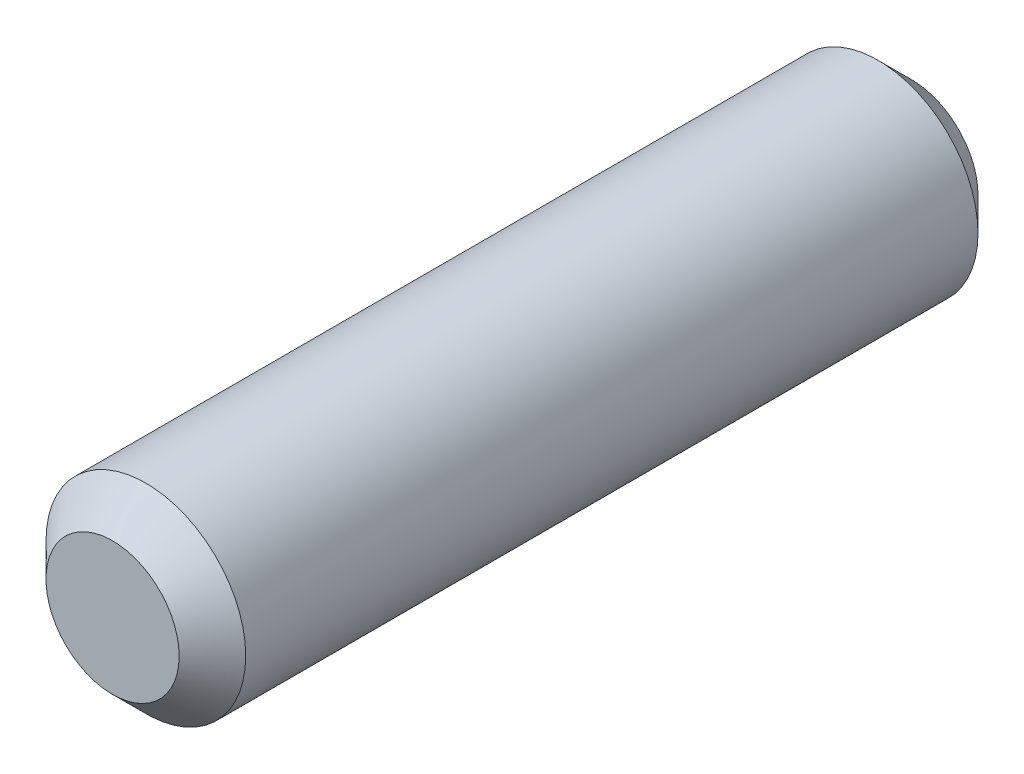
from build123d import *

# Parameters (mm, degrees)
SKETCH1_R           = 3
BOSS_EXTRUDE1_DEPTH = 24
CHAMFER1_SIZE       = 1


with BuildPart() as part:
    # Sketch1 → Boss-Extrude1 (new body)
    with BuildSketch(Plane.XY):
        Circle(SKETCH1_R)
    extrude(amount=BOSS_EXTRUDE1_DEPTH)

    # Chamfer1
    chamfer1_edges = [part.edges().sort_by_distance(p)[0] for p in [
        (-3, 0, 0),
        (-3, 0, 24),
    ]]
    chamfer(chamfer1_edges, length=CHAMFER1_SIZE)


solid = part.part
